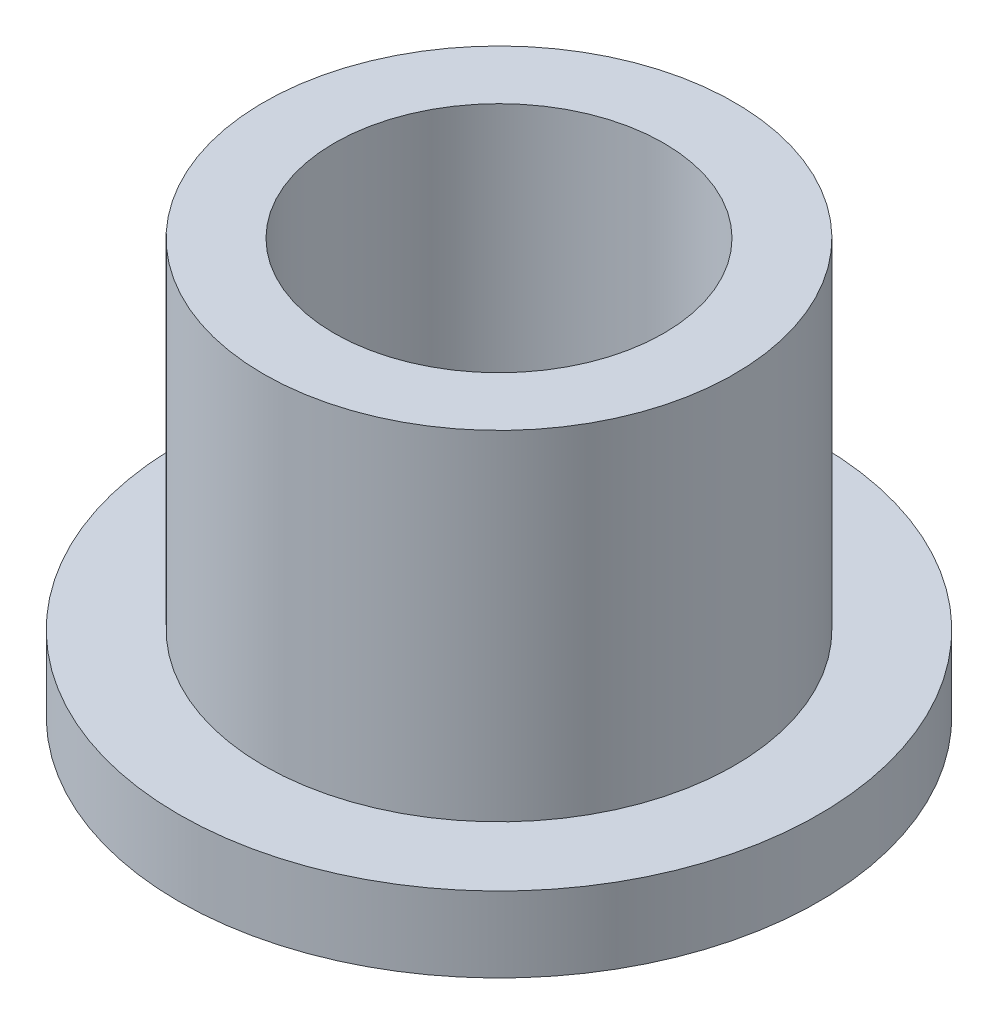
SolidWorks part; units mm, degrees
ref_plane "Front Plane" through (0, 0, 0) normal (0, 0, 1) x (1, 0, 0)
ref_plane "Top Plane" through (0, 0, 0) normal (0, 1, 0) x (1, 0, 0)
ref_plane "Right Plane" through (0, 0, 0) normal (1, 0, 0) x (0, 0, -1)
sketch "Sketch1" plane through (0, 0, 0) normal (0, 1, 0) x (1, 0, 0)
  circle A0 centre (0, 0) radius 34
extrude "Boss-Extrude1" add sketch "Sketch1" along normal blind 8
sketch "Sketch2" plane through (0, 8, 0) normal (0, 1, 0) x (1, 0, 0)
  circle A0 centre (0, 0) radius 25
extrude "Boss-Extrude2" add sketch "Sketch2" along normal blind 36
sketch "Sketch3" plane through (0, 44, 0) normal (0, 1, 0) x (1, 0, 0)
  circle A0 centre (0, 0) radius 17.5
extrude "Cut-Extrude1" cut sketch "Sketch3" against normal through all
